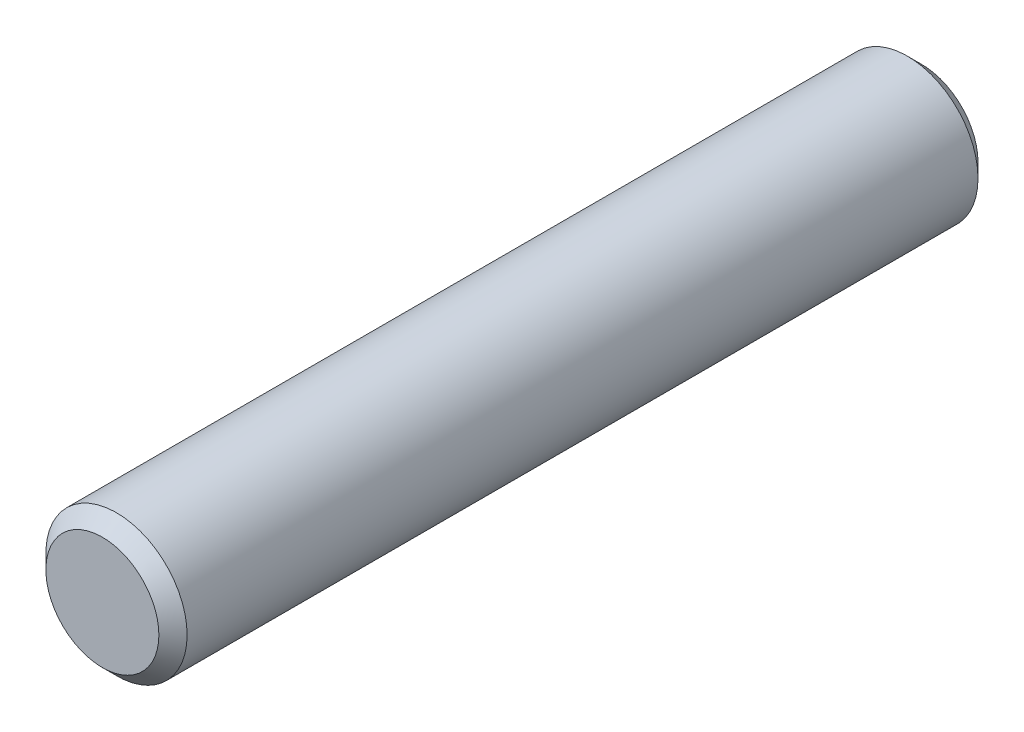
SolidWorks part; units mm, degrees
ref_plane "Front Plane" through (0, 0, 0) normal (0, 0, 1) x (1, 0, 0)
ref_plane "Top Plane" through (0, 0, 0) normal (0, 1, 0) x (1, 0, 0)
ref_plane "Right Plane" through (0, 0, 0) normal (1, 0, 0) x (0, 0, -1)
sketch "Sketch1" plane through (0, 0, 0) normal (0, 0, 1) x (1, 0, 0)
  circle A0 centre (0, 0) radius 0.5
  dimension "D1" = 1
extrude "Boss-Extrude1" add sketch "Sketch1" along normal mid plane 5.8
chamfer "Chamfer1" distance 0.1 angle 45 2 edges at (0.5, 0, -2.9) (0.5, 0, 2.9)
